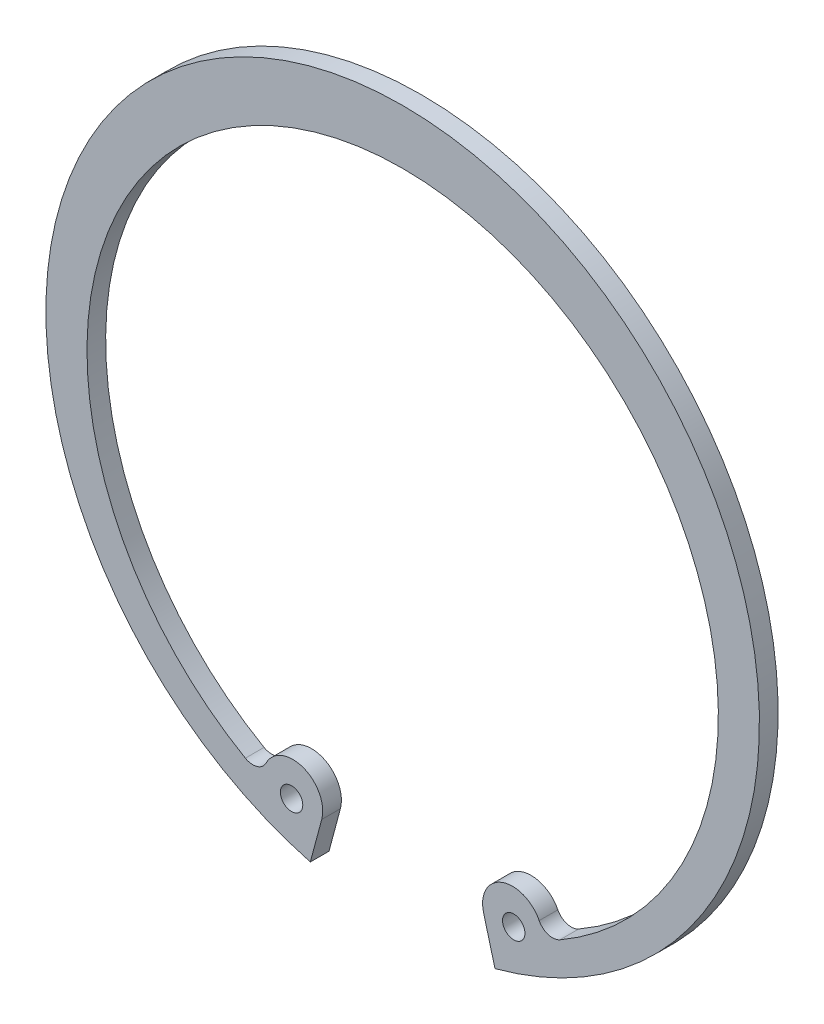
from build123d import *

# Parameters (mm, degrees)
EXTRUDE_962_DEPTH      = 1.25
EXTRUDE_962_DEPTH_BACK = 1.25
SKETCH_1_R             = 1.5


with BuildPart() as part:
    # 草图1 → Extrude 962 (new, two sides: drawn at the far end of the back side and taken through both)
    with BuildSketch(Plane.XY.offset(-EXTRUDE_962_DEPTH_BACK)):
        with BuildLine():
            Line((-10.833988703, -40.432996288), (-12.358609404, -46.122958205))
            ThreePointArc((-12.358609404, -46.122958205), (0, 47.75), (12.358609404, -46.122958205))
            Line((12.358609404, -46.122958205), (10.833988703, -40.432996288))
            ThreePointArc((10.833988703, -40.432996288), (13.272475808, -35.660239835), (18.269709097, -37.597527364))
            ThreePointArc((18.269709097, -37.597527364), (19.48154763, -38.613241212), (21.05227504, -38.43146483))
            ThreePointArc((21.05227504, -38.43146483), (0, 40.45), (-21.05227504, -38.43146483))
            ThreePointArc((-21.05227504, -38.43146483), (-19.48154763, -38.613241212), (-18.269709097, -37.597527364))
            ThreePointArc((-18.269709097, -37.597527364), (-13.272475808, -35.660239835), (-10.833988703, -40.432996288))
        make_face()
        with Locations((-14.866678993, -40.028388123)):
            Circle(SKETCH_1_R, mode=Mode.SUBTRACT)
        with Locations(Location((14.866678993, -40.028388123, 0), (0, 0, 180))):
            Circle(SKETCH_1_R, mode=Mode.SUBTRACT)
    extrude(amount=EXTRUDE_962_DEPTH + EXTRUDE_962_DEPTH_BACK)


solid = part.part
